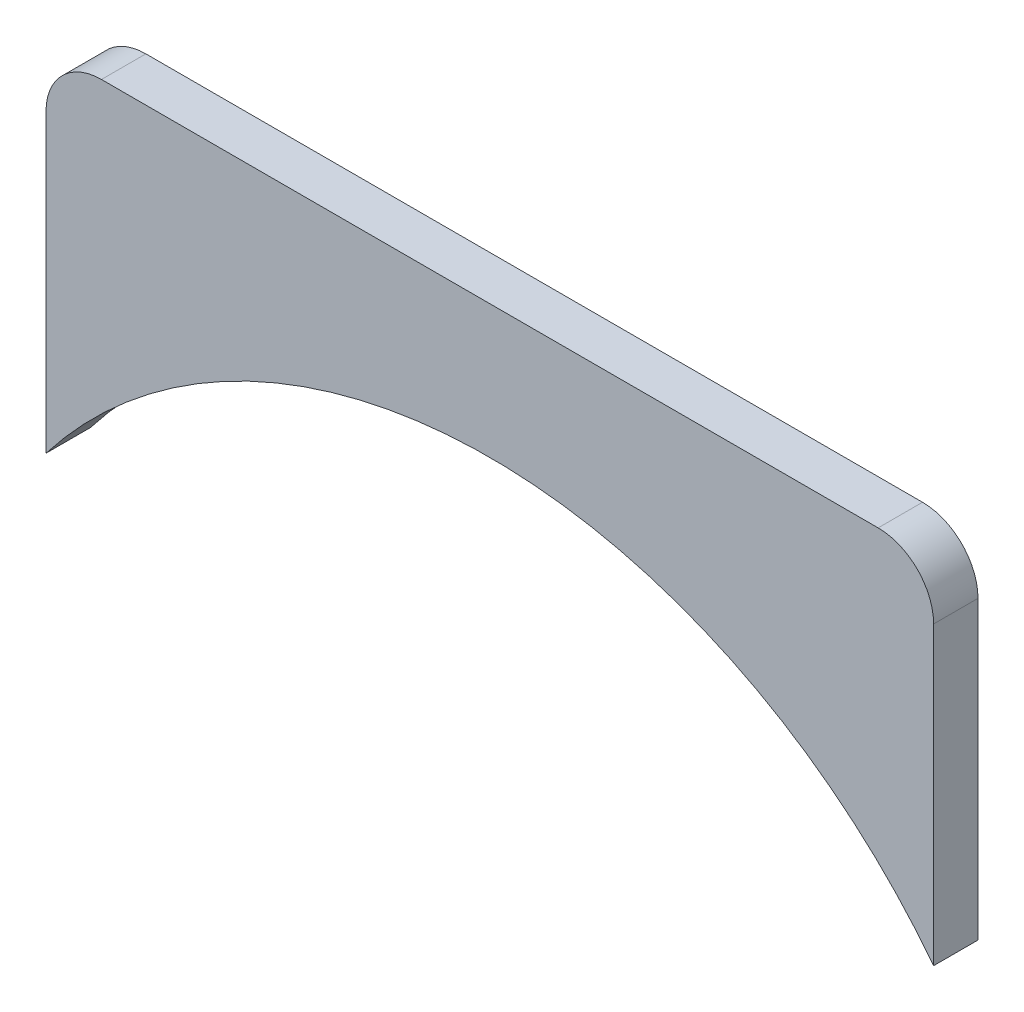
from build123d import *

# Parameters (mm, degrees)
BOSS_EXTRUDE1_DEPTH = 8
FILLET1_R           = 10


with BuildPart() as part:
    # Sketch1 → Boss-Extrude1 (new body)
    with BuildSketch(Plane.XY):
        with BuildLine():
            Line((80, 125), (-80, 125))
            Line((-80, 125), (-80, 61.652250567))
            ThreePointArc((-80, 61.652250567), (0, 101), (80, 61.652250567))
            Line((80, 61.652250567), (80, 125))
        make_face()
    extrude(amount=BOSS_EXTRUDE1_DEPTH)

    # Fillet1
    fillet1_edges = [part.edges().sort_by_distance(p)[0] for p in [
        (-80, 125, 4),
        (80, 125, 4),
    ]]
    fillet(fillet1_edges, radius=FILLET1_R)


solid = part.part
